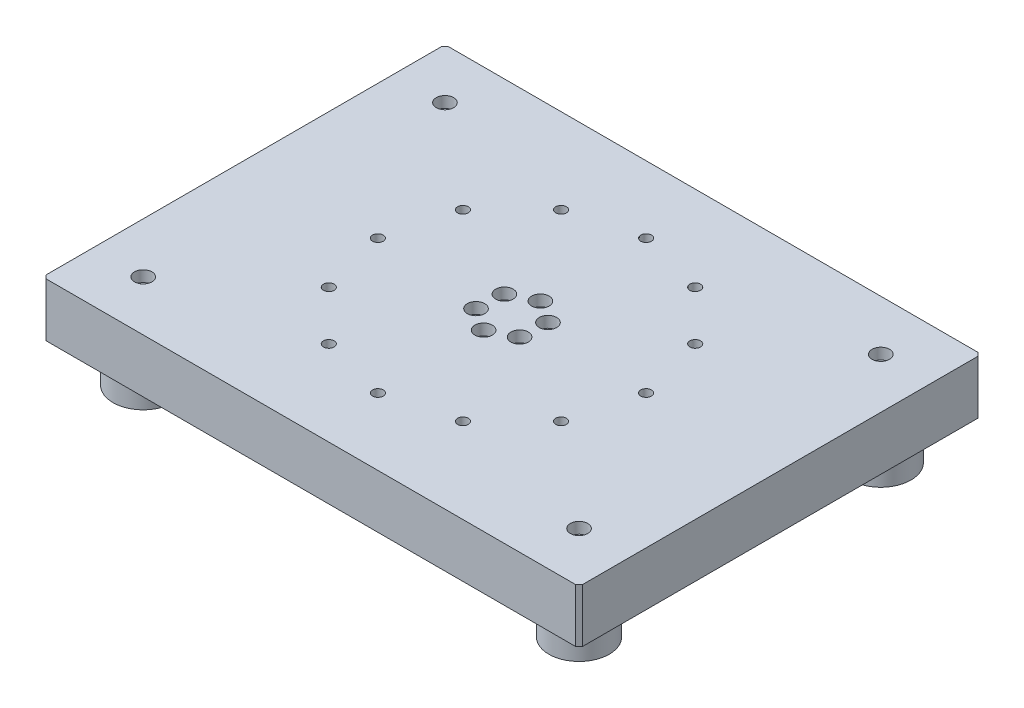
from build123d import *

# Parameters (mm, degrees)
SKETCH1_W                                            = 800
SKETCH1_H                                            = 600
BOSS_EXTRUDE1_DEPTH                                  = 80
CHAMFER1_SIZE                                        = 5
CBORE_FOR_M16_HEX_SOCKET_HEAD_CAP_SCREW1_D           = 17.5
CBORE_FOR_M16_HEX_SOCKET_HEAD_CAP_SCREW1_CBORE_D     = 26
CBORE_FOR_M16_HEX_SOCKET_HEAD_CAP_SCREW1_CBORE_DEPTH = 16.6
SKETCH4_R                                            = 56
CUT_EXTRUDE1_DEPTH                                   = 40
CHAMFER2_SIZE                                        = 5
SKETCH6_R                                            = 45
SKETCH6_R_2                                          = 25
BOSS_EXTRUDE2_DEPTH                                  = 60
CBORE_FOR_M16_HEX_SOCKET_HEAD_CAP_SCREW2_D           = 17.5
CBORE_FOR_M16_HEX_SOCKET_HEAD_CAP_SCREW2_CBORE_D     = 26
CBORE_FOR_M16_HEX_SOCKET_HEAD_CAP_SCREW2_CBORE_DEPTH = 16.6
SKETCH10_R                                           = 8
CUT_EXTRUDE2_DEPTH                                   = 507.359556047
CIRPATTERN1_COUNT                                    = 12


with BuildPart() as part:
    # Sketch1 → Boss-Extrude1 (new body)
    with BuildSketch(Plane(origin=(0, 0, 0), x_dir=(1, 0, 0), z_dir=(0, 1, 0))):
        Rectangle(SKETCH1_W, SKETCH1_H)
    extrude(amount=BOSS_EXTRUDE1_DEPTH)

    # Chamfer1
    chamfer1_edges = [part.edges().sort_by_distance(p)[0] for p in [
        (400, 40, 300),
        (-400, 40, 300),
        (-400, 40, -300),
        (400, 40, -300),
    ]]
    chamfer(chamfer1_edges, length=CHAMFER1_SIZE)

    # CBORE for M16 Hex Socket Head Cap Screw1 (through all)
    with Locations(Plane(origin=(0, 80, 0), x_dir=(1, 0, 0), z_dir=(0, 1, 0))):
        with Locations((2.405406629, 39.927609732), (35.781027655, 17.880661619), (33.375621026, -22.046948113), (-2.405406629, -39.927609732), (-35.781027655, -17.880661619), (-33.375621026, 22.046948113)):
            CounterBoreHole(CBORE_FOR_M16_HEX_SOCKET_HEAD_CAP_SCREW1_D / 2, CBORE_FOR_M16_HEX_SOCKET_HEAD_CAP_SCREW1_CBORE_D / 2, CBORE_FOR_M16_HEX_SOCKET_HEAD_CAP_SCREW1_CBORE_DEPTH)

    # Sketch4 → Cut-Extrude1 (cut)
    with BuildSketch(Plane.XZ):
        with Locations(Location((0, 0, 0), (0, 0, 270))):
            Circle(SKETCH4_R)
    extrude(amount=-CUT_EXTRUDE1_DEPTH, mode=Mode.SUBTRACT)

    # Chamfer2
    chamfer2_edges = [part.edges().sort_by_distance(p)[0] for p in [
        (0, 0, 56),
    ]]
    chamfer(chamfer2_edges, length=CHAMFER2_SIZE)

    # Sketch6 → Boss-Extrude2 (add)
    # profile 1 of 4: a face of its own
    with BuildSketch(Plane.XZ):
        with Locations(Location((-325, 225, 0), (0, 0, 90))):
            Circle(SKETCH6_R)
        with Locations(Location((-325, 225, 0), (0, 0, 270))):
            Circle(SKETCH6_R_2, mode=Mode.SUBTRACT)
    # profile 2 of 4: a face of its own
    with BuildSketch(Plane.XZ):
        with Locations(Location((325, 225, 0), (0, 0, 90))):
            Circle(SKETCH6_R)
        with Locations(Location((325, 225, 0), (0, 0, 270))):
            Circle(SKETCH6_R_2, mode=Mode.SUBTRACT)
    # profile 3 of 4: a face of its own
    with BuildSketch(Plane.XZ):
        with Locations(Location((-325, -225, 0), (0, 0, 90))):
            Circle(SKETCH6_R)
        with Locations(Location((-325, -225, 0), (0, 0, 270))):
            Circle(SKETCH6_R_2, mode=Mode.SUBTRACT)
    # profile 4 of 4: a face of its own
    with BuildSketch(Plane.XZ):
        with Locations(Location((325, -225, 0), (0, 0, 90))):
            Circle(SKETCH6_R)
        with Locations(Location((325, -225, 0), (0, 0, 270))):
            Circle(SKETCH6_R_2, mode=Mode.SUBTRACT)
    extrude(amount=BOSS_EXTRUDE2_DEPTH)

    # CBORE for M16 Hex Socket Head Cap Screw2 (through all)
    with Locations(Plane(origin=(0, 80, 0), x_dir=(1, 0, 0), z_dir=(0, 1, 0))):
        with Locations((-325, -225), (-325, 225), (325, 225), (325, -225)):
            CounterBoreHole(CBORE_FOR_M16_HEX_SOCKET_HEAD_CAP_SCREW2_D / 2, CBORE_FOR_M16_HEX_SOCKET_HEAD_CAP_SCREW2_CBORE_D / 2, CBORE_FOR_M16_HEX_SOCKET_HEAD_CAP_SCREW2_CBORE_DEPTH)

    # Sketch10 → Cut-Extrude2 (cut, through all)
    with BuildSketch(Plane.XZ):
        with Locations(Location((0, 200, 0), (0, 0, 270))):
            Circle(SKETCH10_R)
    cut_extrude2 = extrude(amount=-CUT_EXTRUDE2_DEPTH, mode=Mode.SUBTRACT)

    # CirPattern1: Cut-Extrude2 ×12 about axis
    cirpattern1_axis = Axis((0, 0, 0), (0, 1, 0))
    for i in range(1, CIRPATTERN1_COUNT):
        add(cut_extrude2.rotate(cirpattern1_axis, i * 360 / CIRPATTERN1_COUNT), mode=Mode.SUBTRACT)


solid = part.part
